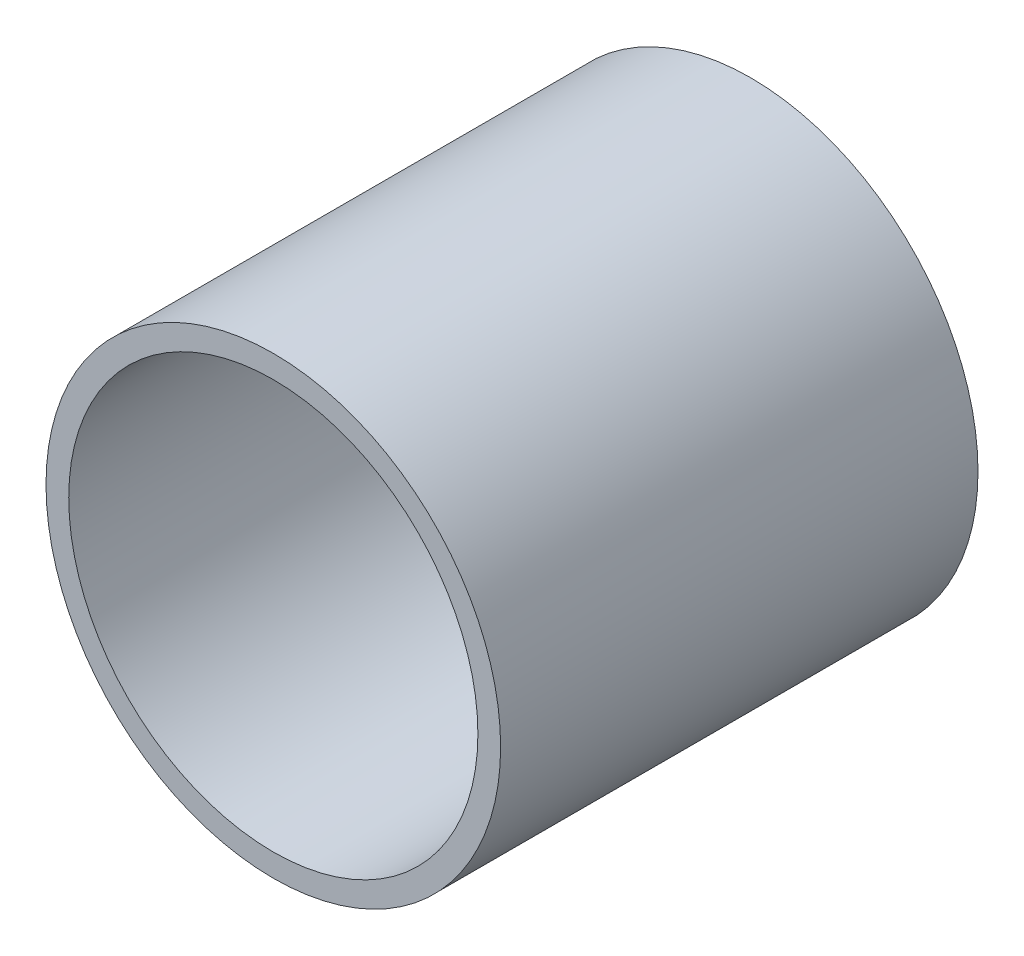
SolidWorks part; units mm, degrees
ref_plane "前视基准面" through (0, 0, 0) normal (0, 0, 1) x (1, 0, 0)
ref_plane "上视基准面" through (0, 0, 0) normal (0, 1, 0) x (1, 0, 0)
ref_plane "右视基准面" through (0, 0, 0) normal (1, 0, 0) x (0, 0, -1)
sketch "草图1" plane through (0, 0, 0) normal (0, 0, 1) x (1, 0, 0)
  circle A0 centre (0, 0) radius 10
  circle A1 centre (0, 0) radius 9
  dimension "D1" = 18
  dimension "D2" = 20
extrude "凸台-拉伸1" add sketch "草图1" along normal blind 21
